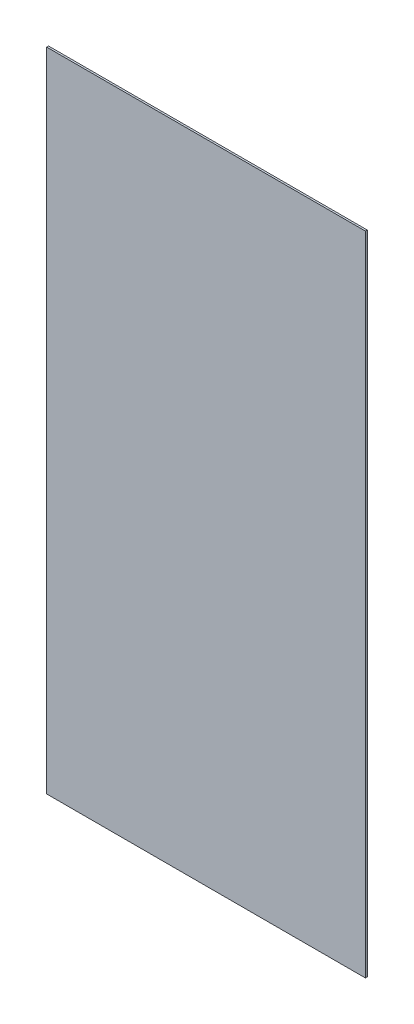
SolidWorks part; units mm, degrees
ref_plane "前视基准面" through (0, 0, 0) normal (0, 0, 1) x (1, 0, 0)
ref_plane "上视基准面" through (0, 0, 0) normal (0, 1, 0) x (1, 0, 0)
ref_plane "右视基准面" through (0, 0, 0) normal (1, 0, 0) x (0, 0, -1)
sketch "草图1" plane through (0, 0, 0) normal (0, 0, 1) x (1, 0, 0)
  line L1 (-251.4024, 170.8841) -> (88.5976, 170.8841)
  line L2 (-251.4024, 170.8841) -> (-251.4024, -519.1159)
  line L3 (-251.4024, -519.1159) -> (88.5976, -519.1159)
  line L4 (88.5976, 170.8841) -> (88.5976, -519.1159)
  dimension "D1" = 690
  dimension "D2" = 340
extrude "凸台-拉伸1" add sketch "草图1" along normal blind 2
